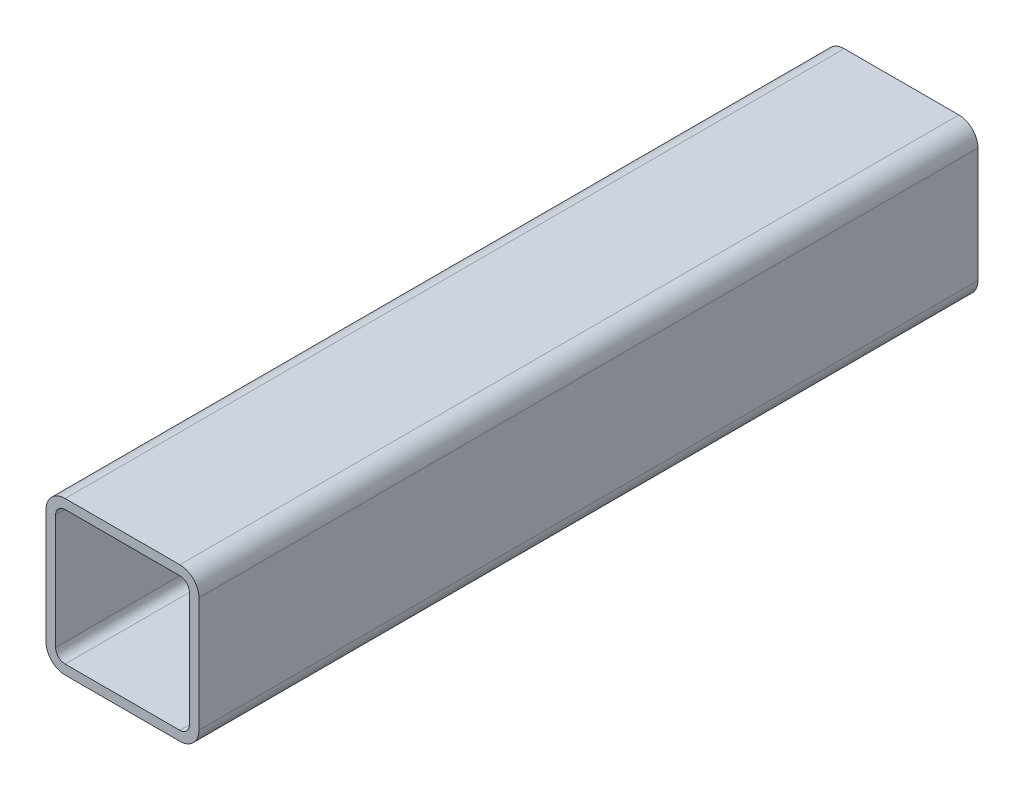
SolidWorks part; units mm, degrees
ref_plane "Front Plane" through (0, 0, 0) normal (0, 0, 1) x (1, 0, 0)
ref_plane "Top Plane" through (0, 0, 0) normal (0, 1, 0) x (1, 0, 0)
ref_plane "Right Plane" through (0, 0, 0) normal (1, 0, 0) x (0, 0, -1)
sketch "Sketch 1" plane through (0, 0, 0) normal (0, 0, 1) x (1, 0, 0)
  line L0 (0, 96.8978) -> (0, -107.4818) construction
  line L1 (-129.1971, 0) -> (137.9562, 0) construction
  line L2 (0, 32) -> (-24, 32)
  line L3 (-32, 24) -> (-32, 0)
  line L4 (0, 28) -> (-24, 28)
  line L5 (-28, 24) -> (-28, 0)
  line L6 (-28, -24) -> (-28, 0)
  line L7 (24, -28) -> (-24, -28)
  line L8 (-32, -24) -> (-32, 0)
  line L9 (24, -32) -> (-24, -32)
  line L10 (32, -24) -> (32, 0)
  line L11 (28, -24) -> (28, 0)
  line L12 (28, 24) -> (28, 0)
  line L13 (0, 28) -> (24, 28)
  line L14 (32, 24) -> (32, 0)
  line L15 (0, 32) -> (24, 32)
  arc A0 (-24, 32) -> (-32, 24) centre (-24, 24) ccw
  arc A1 (-24, 28) -> (-28, 24) centre (-24, 24) ccw
  arc A2 (-24, -28) -> (-28, -24) centre (-24, -24) cw
  arc A3 (-24, -32) -> (-32, -24) centre (-24, -24) cw
  arc A4 (24, -32) -> (32, -24) centre (24, -24) ccw
  arc A5 (24, -28) -> (28, -24) centre (24, -24) ccw
  arc A6 (24, 28) -> (28, 24) centre (24, 24) cw
  arc A7 (24, 32) -> (32, 24) centre (24, 24) cw
  point P34 (0, -32)
  point P35 (0, -28)
  dimension "D3" = 8
  dimension "D1" = 64
  dimension "D2" = 64
  dimension "D4" = 4
extrude "Boss-Extrude 1" add sketch "Sketch 1" along normal mid plane 326
